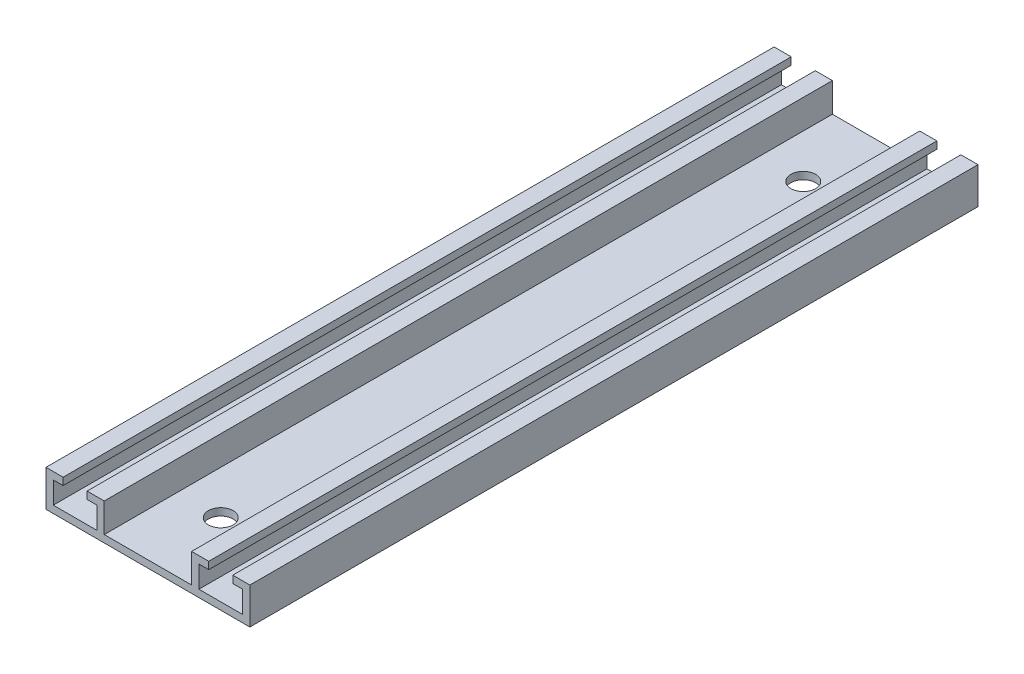
from build123d import *

# Parameters (mm, degrees)
EXTRUDE_1_DEPTH    = 100
SKETCH_2_W         = 6
SKETCH_2_H         = 1
EXTRUDE_2_DEPTH    = 100
HOLE_WIZARD_M3_1_D = 3.4


with BuildPart() as part:
    # 草图1 → 拉伸-薄壁1 (new body)
    with BuildSketch(Plane.XY):
        Polygon((2.35, 5), (0, 5), (0, 0), (8, 0), (8, 5), (5.65, 5), (5.65, 4), (7, 4), (7, 1), (1, 1), (1, 4), (2.35, 4), align=None)
    extrude(amount=EXTRUDE_1_DEPTH)

    # 草图2 → 拉伸-薄壁2 (add)
    with BuildSketch(Plane.XY.offset(100)):
        with Locations((-3, 0.5)):
            Rectangle(SKETCH_2_W, SKETCH_2_H)
    extrude(amount=-EXTRUDE_2_DEPTH)

    # 镜向1: part across plane


with BuildPart() as part_1:
    add(part.part)
    add(part.part.mirror(Plane(origin=(-6, 0, -6.08276253), x_dir=(0, 0, 1), z_dir=(1, 0, 0))))

    # M3 间隙孔1 (through all)
    with Locations(Plane(origin=(0, 1, 0), x_dir=(1, 0, 0), z_dir=(0, 1, 0))):
        with Locations((-6, -90), (-6, -10)):
            Hole(HOLE_WIZARD_M3_1_D / 2)


solid = part_1.part
